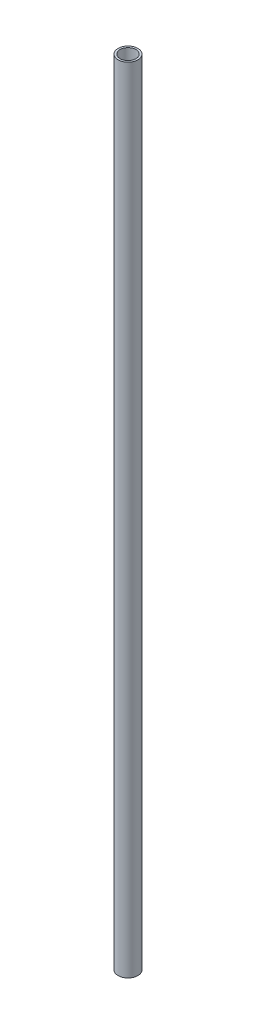
from build123d import *

# Parameters (mm, degrees)
SWEEP_THIN1_PROFILE_R   = 10
SWEEP_THIN1_PROFILE_R_2 = 8


with BuildPart() as part:
    # Sweep-Thin1: sweep along a path in Sketch1
    with BuildLine(Plane.XY) as sweep_thin1_path:
        Line((0, 0), (0, 800))
    # Sweep-Thin1 profile (on start of the path) → Sweep-Thin1 (sweep)
    with BuildSketch(Plane.ZX):
        Circle(SWEEP_THIN1_PROFILE_R)
        Circle(SWEEP_THIN1_PROFILE_R_2, mode=Mode.SUBTRACT)
    sweep(path=sweep_thin1_path.line)


solid = part.part
